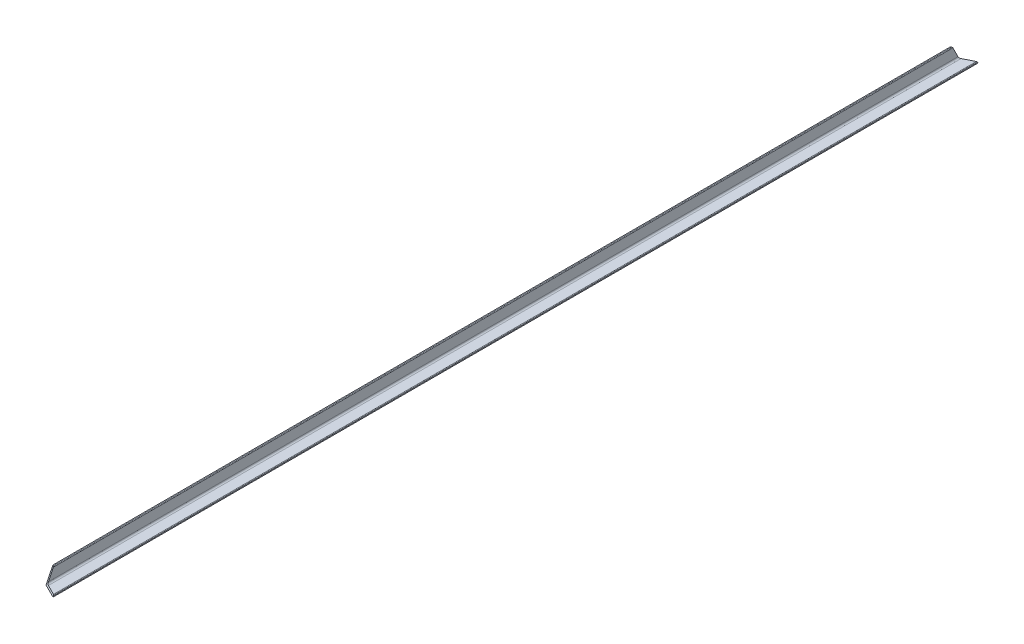
SolidWorks part; units mm, degrees
material "等边角钢70×8/Q235A"
ref_plane "Front Plane" through (0, 0, 0) normal (0, 0, 1) x (1, 0, 0)
ref_plane "Top Plane" through (0, 0, 0) normal (0, 1, 0) x (1, 0, 0)
ref_plane "Right Plane" through (0, 0, 0) normal (1, 0, 0) x (0, 0, -1)
sketch "Sketch1" plane through (0, 0, 0) normal (0, 0, 1) x (1, 0, 0)
  line L0 (0, 70) -> (0, 0)
  line L1 (0, 0) -> (70, 0)
  line L2 (70, 0) -> (70, 5)
  line L3 (67, 8) -> (16, 8)
  line L4 (8, 16) -> (8, 67)
  line L5 (5, 70) -> (0, 70)
  arc A0 (16, 8) -> (8, 16) centre (16, 16) cw
  arc A1 (70, 5) -> (67, 8) centre (67, 5) ccw
  arc A2 (8, 67) -> (5, 70) centre (5, 67) ccw
  dimension "D5" = 8
  dimension "D6" = 3
  dimension "D1" = 70
  dimension "D2" = 70
  dimension "D3" = 8
  dimension "D4" = 8
extrude "Boss-Extrude1" add sketch "Sketch1" along normal blind 4645
ref_plane "Plane1" through (0, 0, 0) normal (0.7071, 0.7071, 0) x (0, 0, -1)
sketch "Sketch3" plane through (0, 0, 0) normal (0.7071, 0.7071, 0) x (0, 0, -1)
  line L0 (0, -49.4975) -> (-69.317, 49.4975)
  line L1 (0, -49.4975) -> (-3, 0) construction
  line L2 (0, 49.4975) -> (0, -49.4975)
  line L3 (-4645, -49.4975) -> (-4645, 49.4975)
  line L4 (-4575.683, 49.4975) -> (-4642, 0) construction
  line L5 (-4575.683, 49.4975) -> (-4645, -49.4975)
  line L6 (0, 49.4975) -> (-69.317, 49.4975)
  line L8 (-4645, 0) -> (0, 0) construction
  line L9 (-3, 0) -> (-69.317, 49.4975) construction
  line L10 (-4645, 49.4975) -> (-4575.683, 49.4975)
  line L12 (-4642, 0) -> (-4645, -49.4975) construction
  dimension "D1" = 35
  dimension "D2" = 35
  dimension "D3" = 3
  dimension "D4" = 3
extrude "Cut-Extrude4" cut sketch "Sketch3" against normal blind 10 and the other way through all
